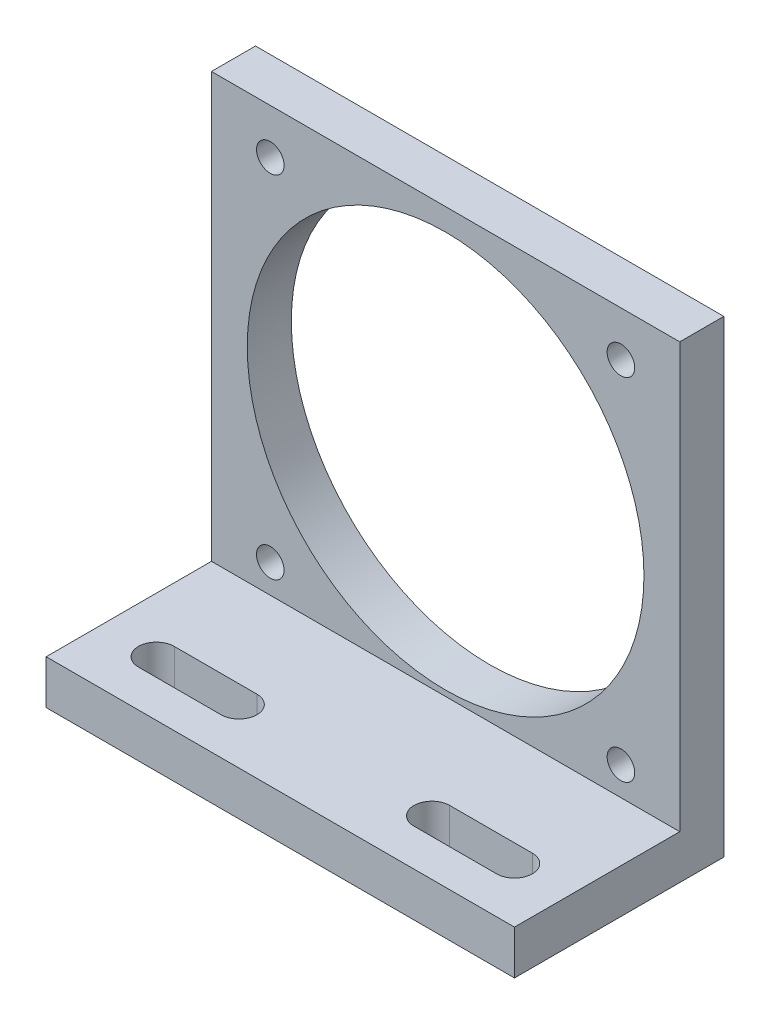
SolidWorks part; units mm, degrees
material "不锈钢 (铁素体)"
ref_plane "前视基准面" through (0, 0, 0) normal (0, 0, 1) x (1, 0, 0)
ref_plane "上视基准面" through (0, 0, 0) normal (0, 1, 0) x (1, 0, 0)
ref_plane "右视基准面" through (0, 0, 0) normal (1, 0, 0) x (0, 0, -1)
sketch "草图1" plane through (0, 0, 0) normal (0, 0, 1) x (1, 0, 0)
  line L1 (-42.5, 42.5) -> (42.5, 42.5)
  line L2 (-42.5, 42.5) -> (-42.5, -42.5)
  line L3 (-42.5, -42.5) -> (42.5, -42.5)
  line L4 (42.5, 42.5) -> (42.5, -42.5)
  line L5 (-42.5, 42.5) -> (42.5, -42.5) construction
  line L6 (-42.5, -42.5) -> (42.5, 42.5) construction
  circle A0 centre (0, 2.5) radius 36
  point P0 (0, 0)
  dimension "D3" = 72
  dimension "D1" = 85
  dimension "D2" = 85
  dimension "D4" = 40
extrude "凸台-拉伸1" add sketch "草图1" along normal mid plane 8
sketch "草图2" plane through (0, 0, 4) normal (0, 0, 1) x (1, 0, 0)
  line L1 (31.8198, -29.3198) -> (-31.8198, -29.3198)
  line L2 (31.8198, -29.3198) -> (31.8198, 34.3198)
  line L3 (31.8198, 34.3198) -> (-31.8198, 34.3198)
  line L4 (-31.8198, -29.3198) -> (-31.8198, 34.3198)
  line L5 (31.8198, -29.3198) -> (-31.8198, 34.3198) construction
  line L6 (31.8198, 34.3198) -> (-31.8198, -29.3198) construction
  point P0 (0, 2.5)
  dimension "D1" = 90
hole_wizard "M6 螺纹孔1" positions "3D草图1" profile "草图3" tap size "M6" standard "GB" end condition through all
sketch3d "3D草图1"
  point P0 (-31.8198, 34.3198, 4)
  point P7 (31.8198, -29.3198, 4)
  point P10 (-31.8198, -29.3198, 4)
  point P13 (31.8198, 34.3198, 4)
sketch "草图3" plane through (-31.8198, 34.3198, 4) normal (1, 0, 0) x (0, -1, 0)
  line L0 (0, 0) -> (0, 8)
  line L1 (0, 8) -> (2.5, 8)
  line L2 (2.5, 8) -> (2.5, 0)
  line L5 (2.5, 0) -> (0, 0)
  line L11 (0, -6.35) -> (0, 107.95) construction
  dimension "通孔螺纹孔钻头直径" = 5
  dimension "通孔螺纹孔钻头深度" = 8
cosmetic thread "孔螺蚊线1" parameters "D2"=6
cosmetic thread "孔螺蚊线2" parameters "D2"=6
cosmetic thread "孔螺蚊线3" parameters "D2"=6
cosmetic thread "孔螺蚊线4" parameters "D2"=6
sketch "草图4" plane through (0, 0, 4) normal (0, 0, 1) x (1, 0, 0)
  line L0 (42.5, -42.5) -> (42.5, 42.5) construction
  line L1 (-42.5, -42.5) -> (42.5, -42.5)
  line L2 (-42.5, -42.5) -> (-42.5, -34.5)
  line L3 (-42.5, -34.5) -> (42.5, -34.5)
  line L4 (42.5, -42.5) -> (42.5, -34.5)
  dimension "D1" = 8
extrude "凸台-拉伸2" add sketch "草图4" along normal blind 30
sketch "草图5" plane through (0, -34.5, 0) normal (0, 1, 0) x (1, 0, 0)
  line L0 (-32.5, -24) -> (-17.5, -24) construction
  line L1 (-32.5, -20.75) -> (-17.5, -20.75)
  line L2 (-32.5, -27.25) -> (-17.5, -27.25)
  line L3 (17.5, -24) -> (32.5, -24) construction
  line L4 (17.5, -20.75) -> (32.5, -20.75)
  line L5 (17.5, -27.25) -> (32.5, -27.25)
  line L6 (-42.5, -34) -> (-42.5, -4) construction
  line L7 (42.5, -34) -> (42.5, -4) construction
  line L9 (42.5, -34) -> (-42.5, -34) construction
  arc A0 (-32.5, -20.75) -> (-32.5, -27.25) centre (-32.5, -24) ccw
  arc A1 (-17.5, -27.25) -> (-17.5, -20.75) centre (-17.5, -24) ccw
  arc A2 (17.5, -20.75) -> (17.5, -27.25) centre (17.5, -24) ccw
  arc A3 (32.5, -27.25) -> (32.5, -20.75) centre (32.5, -24) ccw
  point P2 (-25, -24)
  point P7 (25, -24)
  dimension "D1" = 6.5
  dimension "D2" = 15
  dimension "D3" = 10
  dimension "D4" = 10
  dimension "D5" = 10
extrude "切除-拉伸1" cut sketch "草图5" against normal through all
